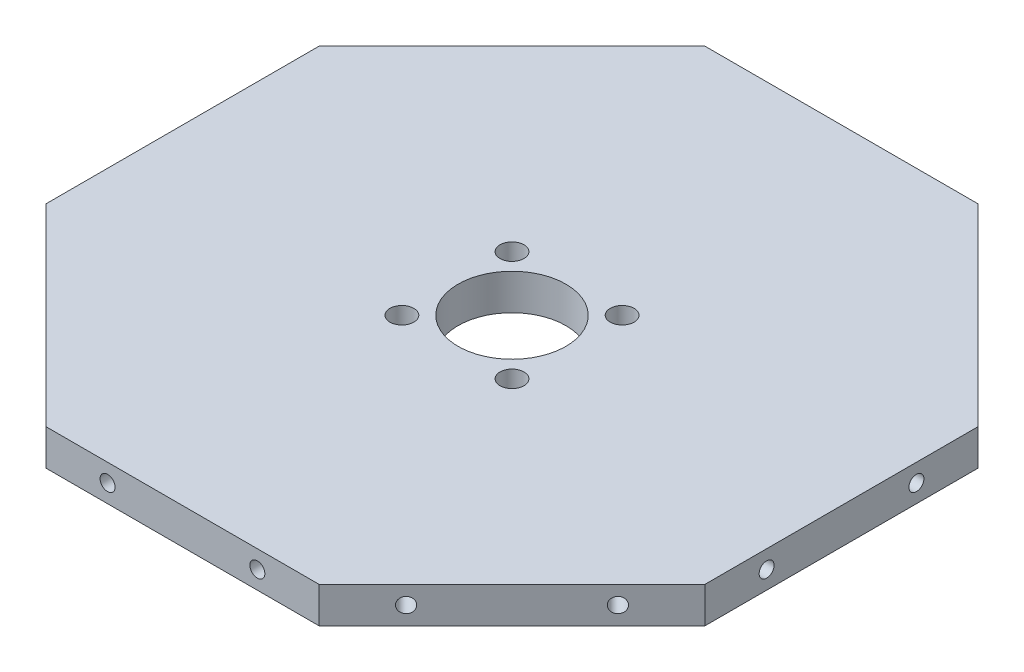
from build123d import *

# Parameters (mm, degrees)
SKETCH_1_W               = 102
SKETCH_1_H               = 12
CUT_EXTRUDE_1_DEPTH      = 83
M6X1_0_1_AT_2_COUNT      = 2
M6X1_0_1_AT_2_PITCH      = 50
PATTERN_CIRCULAR_1_COUNT = 8
SKETCH_7_R               = 1.65
CUT_EXTRUDE_2_DEPTH      = 30
SKETCH_8_R               = 4
CUT_EXTRUDE_3_DEPTH      = 7
PATTERN_CIRCULAR_2_COUNT = 4


with BuildPart() as part:
    # 草图1 → 旋转1 (revolve)
    with BuildSketch(Plane.XY, mode=Mode.PRIVATE) as revolve_1_sk:
        with Locations((69, 0)):
            Rectangle(SKETCH_1_W, SKETCH_1_H)
    revolve(revolve_1_sk.sketch.rotate(Axis((0, 0, 0), (0, 1, 0)), 90), axis=Axis((0, 0, 0), (0, 1, 0)))

    # 草图4 → 切除-拉伸1 (cut)
    with BuildSketch(Plane(origin=(0, 6, 0), x_dir=(1, 0, 0), z_dir=(0, 1, 0))):
        Polygon((110, 627.554648283), (110, 47.958315233), (110, -47.958315233), (110, -627.554648283), (1269.1926661, -627.554648283), (1269.1926661, 627.554648283), align=None)
    cut_extrude_1 = extrude(amount=-CUT_EXTRUDE_1_DEPTH, mode=Mode.SUBTRACT)

    # 草图6 → M6x1.0 螺纹孔1 (revolve, cut)
    with BuildSketch(Plane(origin=(110, 0, 25), x_dir=(0, 0, -1), z_dir=(0, 1, 0))):
        Polygon((0, 0), (0, 13.502151548), (2.5, 12), (2.5, 0), align=None)
    m6x1_0_1 = revolve(axis=Axis((116.35, 0, 25), (-1, 0, 0)), mode=Mode.SUBTRACT)

    # M6x1.0 螺纹孔1 at 2: M6x1.0 螺纹孔1 ×2
    with Locations(*[(0, 0, -i * M6X1_0_1_AT_2_PITCH) for i in range(1, M6X1_0_1_AT_2_COUNT)]):
        add(m6x1_0_1, mode=Mode.SUBTRACT)

    # 阵列(圆周)1: 切除-拉伸1, M6x1.0 螺纹孔1 ×8 about axis
    pattern_circular_1_axis = Axis((0, 0, 0), (0, 1, 0))
    add([cut_extrude_1.rotate(pattern_circular_1_axis, i * 360 / PATTERN_CIRCULAR_1_COUNT) for i in range(1, PATTERN_CIRCULAR_1_COUNT)], mode=Mode.SUBTRACT)
    add([m6x1_0_1.rotate(pattern_circular_1_axis, i * 360 / PATTERN_CIRCULAR_1_COUNT) for i in range(1, PATTERN_CIRCULAR_1_COUNT)], mode=Mode.SUBTRACT)

    # 阵列(圆周)1 copy 1 sketch → 阵列(圆周)1 copy 1 (revolve, cut)
    with BuildSketch(Plane(origin=(60.104076401, 0, -95.45941546), x_dir=(-0.7071067811865475, 0, -0.7071067811865476), z_dir=(0, 1, 0))):
        Polygon((0, 0), (0, 13.502151548), (2.5, 12), (2.5, 0), align=None)
    revolve(axis=Axis((64.594204461, 0, -99.949543521), (-0.7071067811865476, 0, 0.7071067811865475)), mode=Mode.SUBTRACT)

    # 阵列(圆周)1 copy 2 sketch → 阵列(圆周)1 copy 2 (revolve, cut)
    with BuildSketch(Plane(origin=(-25, 0, -110), x_dir=(-1, 0, 0), z_dir=(0, 1, 0))):
        Polygon((0, 0), (0, 13.502151548), (2.5, 12), (2.5, 0), align=None)
    revolve(axis=Axis((-25, 0, -116.35), (0, 0, 1)), mode=Mode.SUBTRACT)

    # 阵列(圆周)1 copy 3 sketch → 阵列(圆周)1 copy 3 (revolve, cut)
    with BuildSketch(Plane(origin=(-95.45941546, 0, -60.104076401), x_dir=(-0.7071067811865476, 0, 0.7071067811865475), z_dir=(0, 1, 0))):
        Polygon((0, 0), (0, 13.502151548), (2.5, 12), (2.5, 0), align=None)
    revolve(axis=Axis((-99.949543521, 0, -64.594204461), (0.7071067811865475, 0, 0.7071067811865476)), mode=Mode.SUBTRACT)

    # 阵列(圆周)1 copy 4 sketch → 阵列(圆周)1 copy 4 (revolve, cut)
    with BuildSketch(Plane(origin=(-110, 0, 25), x_dir=(0, 0, 1), z_dir=(0, 1, 0))):
        Polygon((0, 0), (0, 13.502151548), (2.5, 12), (2.5, 0), align=None)
    revolve(axis=Axis((-116.35, 0, 25), (1, 0, 0)), mode=Mode.SUBTRACT)

    # 阵列(圆周)1 copy 5 sketch → 阵列(圆周)1 copy 5 (revolve, cut)
    with BuildSketch(Plane(origin=(-60.104076401, 0, 95.45941546), x_dir=(0.7071067811865475, 0, 0.7071067811865477), z_dir=(0, 1, 0))):
        Polygon((0, 0), (0, 13.502151548), (2.5, 12), (2.5, 0), align=None)
    revolve(axis=Axis((-64.594204461, 0, 99.949543521), (0.7071067811865477, 0, -0.7071067811865475)), mode=Mode.SUBTRACT)

    # 阵列(圆周)1 copy 6 sketch → 阵列(圆周)1 copy 6 (revolve, cut)
    with BuildSketch(Plane(origin=(25, 0, 110), x_dir=(1, 0, 0), z_dir=(0, 1, 0))):
        Polygon((0, 0), (0, 13.502151548), (2.5, 12), (2.5, 0), align=None)
    revolve(axis=Axis((25, 0, 116.35), (0, 0, -1)), mode=Mode.SUBTRACT)

    # 阵列(圆周)1 copy 7 sketch → 阵列(圆周)1 copy 7 (revolve, cut)
    with BuildSketch(Plane(origin=(95.45941546, 0, 60.104076401), x_dir=(0.7071067811865477, 0, -0.7071067811865474), z_dir=(0, 1, 0))):
        Polygon((0, 0), (0, 13.502151548), (2.5, 12), (2.5, 0), align=None)
    revolve(axis=Axis((99.949543521, 0, 64.594204461), (-0.7071067811865474, 0, -0.7071067811865477)), mode=Mode.SUBTRACT)

    # 草图7 → 切除-拉伸2 (cut)
    with BuildSketch(Plane(origin=(0, 6, 0), x_dir=(1, 0, 0), z_dir=(0, 1, 0))):
        with Locations(Location((18.384776311, 18.384776311, 0), (0, 0, 270))):
            Circle(SKETCH_7_R)
    cut_extrude_2 = extrude(amount=-CUT_EXTRUDE_2_DEPTH, mode=Mode.SUBTRACT)

    # 草图8 → 切除-拉伸3 (cut)
    with BuildSketch(Plane(origin=(0, 6, 0), x_dir=(1, 0, 0), z_dir=(0, 1, 0))):
        with Locations(Location((18.384776311, 18.384776311, 0), (0, 0, 270))):
            Circle(SKETCH_8_R)
    cut_extrude_3 = extrude(amount=-CUT_EXTRUDE_3_DEPTH, mode=Mode.SUBTRACT)

    # 阵列(圆周)2: 切除-拉伸2, 切除-拉伸3 ×4 about axis
    pattern_circular_2_axis = Axis((0, 0, 0), (0, 1, 0))
    add([cut_extrude_2.rotate(pattern_circular_2_axis, i * 360 / PATTERN_CIRCULAR_2_COUNT) for i in range(1, PATTERN_CIRCULAR_2_COUNT)], mode=Mode.SUBTRACT)
    add([cut_extrude_3.rotate(pattern_circular_2_axis, i * 360 / PATTERN_CIRCULAR_2_COUNT) for i in range(1, PATTERN_CIRCULAR_2_COUNT)], mode=Mode.SUBTRACT)


solid = part.part
